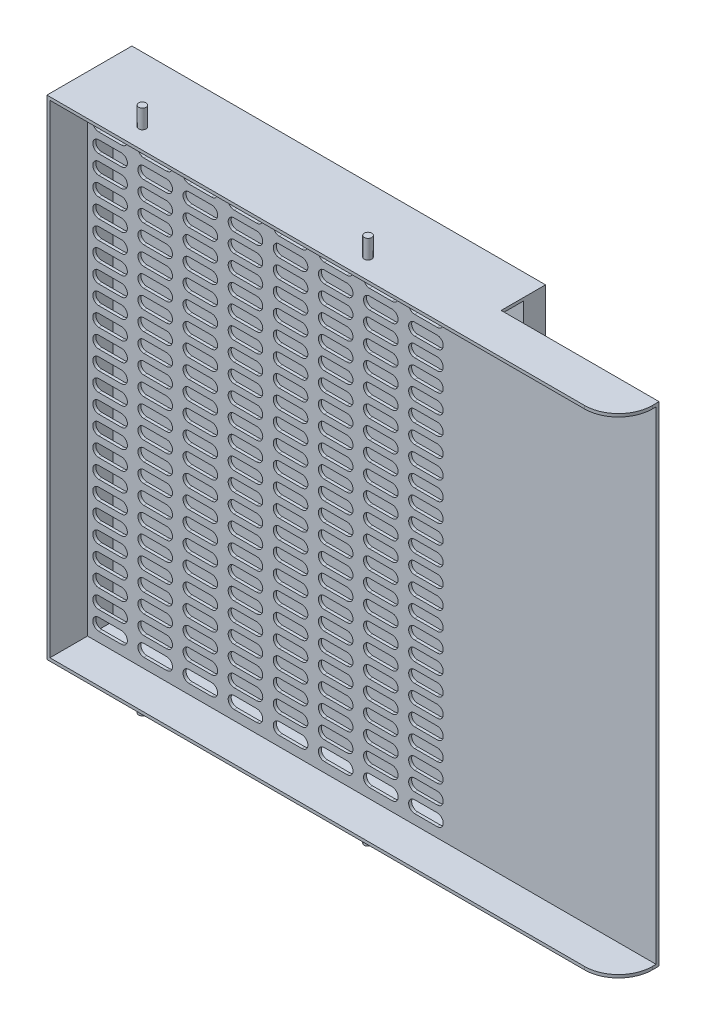
SolidWorks part; units mm, degrees
material "AISI 304"
ref_plane "Front Plane" through (0, 0, 0) normal (0, 0, 1) x (1, 0, 0)
ref_plane "Top Plane" through (0, 0, 0) normal (0, 1, 0) x (1, 0, 0)
ref_plane "Right Plane" through (0, 0, 0) normal (1, 0, 0) x (0, 0, -1)
other "Configuration Table"
sketch "Sketch1" plane through (0, 0, 0) normal (0, 0, 1) x (1, 0, 0)
  line L1 (-250, 325) -> (250, 325)
  line L2 (-250, 325) -> (-250, -325)
  line L3 (-250, -325) -> (250, -325)
  line L4 (250, 325) -> (250, -325)
  line L5 (-250, 325) -> (250, -325) construction
  line L6 (-250, -325) -> (250, 325) construction
  point P0 (0, 0)
  dimension "D1" = 500
  dimension "D2" = 650
extrude "Boss-Extrude1" add sketch "Sketch1" along normal mid plane 4
sketch "Sketch2" plane through (0, 0, 2) normal (0, 0, 1) x (1, 0, 0)
  line L0 (-246, 321) -> (-246, -321)
  line L1 (-246, -321) -> (246, -321)
  line L2 (246, -321) -> (246, 321)
  line L3 (246, 321) -> (-246, 321)
  line L4 (250, -325) -> (250, 325)
  line L5 (250, 325) -> (-250, 325)
  line L6 (-250, 325) -> (-250, -325)
  line L7 (-250, -325) -> (250, -325)
  line L8 (250, -325) -> (250, 325)
  line L9 (250, 325) -> (-250, 325)
  line L10 (-250, 325) -> (-250, -325)
  line L11 (-250, -325) -> (250, -325)
  dimension "D2" = 4
  dimension "D1" = 0
extrude "Boss-Extrude2" add sketch "Sketch2" along normal blind 50
sketch "Sketch3" plane through (0, -325, 0) normal (0, -1, 0) x (1, 0, 0)
  line L0 (-250, 25) -> (250, 25) construction
  line L1 (-250, 52) -> (-250, -2) construction
  line L2 (250, 52) -> (250, -2) construction
  circle A0 centre (150, 25) radius 5
  circle A1 centre (-150, 25) radius 5
  dimension "D1" = 10
  dimension "D2" = 10
  dimension "D3" = 100
  dimension "D4" = 300
extrude "Boss-Extrude3" add sketch "Sketch3" along normal blind 25
sketch "Sketch4" plane through (0, 325, 0) normal (0, 1, 0) x (1, 0, 0)
  line L0 (250, -25) -> (-250, -25) construction
  line L1 (250, -52) -> (250, 2) construction
  line L2 (-250, -52) -> (-250, 2) construction
  circle A0 centre (150, -25) radius 5
  circle A1 centre (-150, -25) radius 5
  dimension "D1" = 10
  dimension "D2" = 10
  dimension "D3" = 300
  dimension "D4" = 100
extrude "Boss-Extrude4" add sketch "Sketch4" along normal blind 25
sketch "Sketch5" plane through (246, 0, 0) normal (-1, 0, 0) x (0, 0, 1)
  line L4 (2, 321) -> (2, -321)
  line L5 (2, -321) -> (52, -321)
  line L6 (52, -321) -> (52, 321)
  line L7 (52, 321) -> (2, 321)
  line L8 (2, 321) -> (2, -321)
  line L9 (2, -321) -> (52, -321)
  line L10 (52, -321) -> (52, 321)
  line L11 (52, 321) -> (2, 321)
  dimension "D1" = 0
extrude "Cut-Extrude1" cut sketch "Sketch5" against normal blind 25
sketch "Sketch6" plane through (250, 0, 0) normal (1, 0, 0) x (0, 0, -1)
  line L8 (-52, 325) -> (-52, 321)
  line L9 (-52, 321) -> (-2, 321)
  line L10 (-2, 321) -> (-2, -321)
  line L11 (-2, -321) -> (-52, -321)
  line L12 (-52, -321) -> (-52, -325)
  line L13 (-52, -325) -> (2, -325)
  line L14 (2, -325) -> (2, 325)
  line L15 (2, 325) -> (-52, 325)
  line L16 (-52, 325) -> (-52, 321)
  line L17 (-52, 321) -> (-2, 321)
  line L18 (-2, 321) -> (-2, -321)
  line L19 (-2, -321) -> (-52, -321)
  line L20 (-52, -321) -> (-52, -325)
  line L21 (-52, -325) -> (2, -325)
  line L22 (2, -325) -> (2, 325)
  line L23 (2, 325) -> (-52, 325)
  dimension "D1" = 0
extrude "Boss-Extrude5" add sketch "Sketch6" along normal blind 50
sketch "Sketch9" plane through (0, 0, -2) normal (0, 0, -1) x (-1, 0, 0)
  line L0 (-296, 321) -> (-296, -321)
  line L1 (-296, -321) -> (246, -321)
  line L2 (246, -321) -> (246, 321)
  line L3 (246, 321) -> (-296, 321)
  line L4 (250, 325) -> (-300, 325)
  line L5 (-300, 325) -> (-300, -325)
  line L6 (-300, -325) -> (250, -325)
  line L7 (250, -325) -> (250, 325)
  line L8 (250, 325) -> (-300, 325)
  line L9 (-300, 325) -> (-300, -325)
  line L10 (-300, -325) -> (250, -325)
  line L11 (250, -325) -> (250, 325)
  line L12 (-296, 321) -> (-300, 321)
  line L13 (-296, -321) -> (-300, -321)
  line M9 (250, 325) -> (-300, 325)
  line M10 (-300, 325) -> (-300, -325)
  line M11 (-300, -325) -> (250, -325)
  line M12 (250, -325) -> (250, 325)
  dimension "D1" = 0
  dimension "D2" = 4
extrude "Boss-Extrude7" add sketch "Sketch9" along normal blind 30 contours L1 L13 L12 L3 L2 M10 M11 M12 M9
sketch "Sketch10" plane through (0, 0, -32) normal (0, 0, -1) x (-1, 0, 0)
  line L1 (-300, 325) -> (250, 325)
  line L2 (-300, 325) -> (-300, -325)
  line L3 (-300, -325) -> (250, -325)
  line L4 (250, 325) -> (250, -325)
extrude "Boss-Extrude8" add sketch "Sketch10" along normal blind 4
sketch "Sketch11" plane through (0, 0, 2) normal (0, 0, 1) x (1, 0, 0)
  line L0 (-246, 0) -> (300, 0) construction
  line L1 (-246, 321) -> (-246, -321) construction
  line L2 (300, 321) -> (300, -321) construction
  line L3 (-231, 0) -> (-201, 0) construction
  line L4 (-231, 8) -> (-201, 8)
  line L5 (-231, -8) -> (-201, -8)
  line L6 (-171, 0) -> (-141, 0) construction
  line L7 (-171, 8) -> (-141, 8)
  line L8 (-171, -8) -> (-141, -8)
  line L9 (-111, 0) -> (-81, 0) construction
  line L10 (-111, 8) -> (-81, 8)
  line L11 (-111, -8) -> (-81, -8)
  line L12 (-51, 0) -> (-21, 0) construction
  line L13 (-51, 8) -> (-21, 8)
  line L14 (-51, -8) -> (-21, -8)
  line L15 (9, 0) -> (39, 0) construction
  line L16 (9, 8) -> (39, 8)
  line L17 (9, -8) -> (39, -8)
  line L18 (69, 0) -> (99, 0) construction
  line L19 (69, 8) -> (99, 8)
  line L20 (69, -8) -> (99, -8)
  line L21 (129, 0) -> (159, 0) construction
  line L22 (129, 8) -> (159, 8)
  line L23 (129, -8) -> (159, -8)
  line L24 (189, 0) -> (219, 0) construction
  line L25 (189, 8) -> (219, 8)
  line L26 (189, -8) -> (219, -8)
  arc A0 (-231, 8) -> (-231, -8) centre (-231, 0) ccw
  arc A1 (-201, -8) -> (-201, 8) centre (-201, 0) ccw
  arc A2 (-171, 8) -> (-171, -8) centre (-171, 0) ccw
  arc A3 (-141, -8) -> (-141, 8) centre (-141, 0) ccw
  arc A4 (-111, 8) -> (-111, -8) centre (-111, 0) ccw
  arc A5 (-81, -8) -> (-81, 8) centre (-81, 0) ccw
  arc A6 (-51, 8) -> (-51, -8) centre (-51, 0) ccw
  arc A7 (-21, -8) -> (-21, 8) centre (-21, 0) ccw
  arc A8 (9, 8) -> (9, -8) centre (9, 0) ccw
  arc A9 (39, -8) -> (39, 8) centre (39, 0) ccw
  arc A10 (69, 8) -> (69, -8) centre (69, 0) ccw
  arc A11 (99, -8) -> (99, 8) centre (99, 0) ccw
  arc A12 (129, 8) -> (129, -8) centre (129, 0) ccw
  arc A13 (159, -8) -> (159, 8) centre (159, 0) ccw
  arc A14 (189, 8) -> (189, -8) centre (189, 0) ccw
  arc A15 (219, -8) -> (219, 8) centre (219, 0) ccw
  point P8 (-216, 0)
  point P16 (-156, 0)
  point P23 (-96, 0)
  point P30 (-36, 0)
  point P37 (24, 0)
  point P44 (84, 0)
  point P51 (144, 0)
  point P58 (204, 0)
  dimension "D2" = 8
  dimension "D1" = 30
  dimension "D3" = 15
  dimension "D4" = 8
extrude "Cut-Extrude3" cut sketch "Sketch11" against normal blind 4
pattern_linear "LPattern1" count 13 spacing 25 along (0, -1, 0) of "Cut-Extrude3"
pattern_linear "LPattern2" count 13 spacing 25 along (0, 1, 0) of "Cut-Extrude3"
sketch "Sketch13" plane through (0, 0, -36) normal (0, 0, -1) x (-1, 0, 0)
  line L0 (-275, 300) -> (-275, -300)
  line L1 (-275, -300) -> (225, -300)
  line L2 (225, -300) -> (225, 300)
  line L3 (225, 300) -> (-275, 300)
  line L4 (-300, 325) -> (-300, -325)
  line L5 (-300, -325) -> (250, -325)
  line L6 (250, -325) -> (250, 325)
  line L7 (250, 325) -> (-300, 325)
  line L8 (-300, 325) -> (-300, -325)
  line L9 (-300, -325) -> (250, -325)
  line L10 (250, -325) -> (250, 325)
  line L11 (250, 325) -> (-300, 325)
  line L13 (300, 31.3075) -> (-300, 31.3075)
  line L14 (300, 31.3075) -> (300, -31.3075)
  line L15 (300, -31.3075) -> (-300, -31.3075)
  line L16 (-300, 31.3075) -> (-300, -31.3075)
  line L17 (300, 31.3075) -> (-300, -31.3075) construction
  line L18 (300, -31.3075) -> (-300, 31.3075) construction
  line L19 (305.8934, 6.3075) -> (-300, 6.3075)
  line L20 (305.8934, 6.3075) -> (305.8934, -5.6925)
  line L21 (305.8934, -5.6925) -> (-300, -5.6925)
  line L22 (-300, 6.3075) -> (-300, -5.6925)
  line L23 (305.8934, 6.3075) -> (-300, -5.6925) construction
  line L24 (305.8934, -5.6925) -> (-300, 6.3075) construction
  point P8 (0, 0)
  point P13 (2.9467, 0.3075)
  line M15 (-300, 325) -> (-300, -325)
  line M16 (-300, -325) -> (250, -325)
  line M17 (250, -325) -> (250, 325)
  line M18 (250, 325) -> (-300, 325)
  dimension "D3" = 25
  dimension "D4" = 605.8934
  dimension "D5" = 12
  dimension "D1" = 0
  dimension "D2" = 25
extrude "Boss-Extrude10" add sketch "Sketch13" along normal blind 25 contours L13 L10 L0 L3 L2 M18 M15 | L19 L2 L13 L0 | L2 L21 L0 L15 | L0 L21 L8 L15 | L19 L0 L13 L8 | L15 L2 L1 L0 M17 M15 M16 | L21 L0 L19 L16 | L10 L21 L2 L15 | L21 L19 L2 M17 | L19 L13 L2 M17
sketch "Sketch14" plane through (0, 0, 0) normal (0, 1, 0) x (1, 0, 0)
  line L0 (-250, 48.5) -> (300, 48.5) construction
  line L1 (-250, -52) -> (-250, 61) construction
  line L2 (300, 61) -> (300, -52) construction
  line L3 (-250, 61) -> (300, 61) construction
  circle A0 centre (25, 48.5) radius 5
  dimension "D2" = 10
  dimension "D1" = 12.5
extrude "Cut-Extrude4" cut sketch "Sketch14" against normal mid plane 80
sketch "Sketch15" plane through (300, 0, 0) normal (1, 0, 0) x (0, 0, -1)
  line L0 (2, 321) -> (2, -325)
  line L1 (2, -325) -> (-52, -325)
  line L2 (2, 320.1324) -> (2, 325)
  line L3 (2, 325) -> (-52, 325)
  line L8 (-52, -325) -> (61, -325)
  line L9 (61, -325) -> (61, 325)
  line L10 (61, 325) -> (-52, 325)
  line L11 (-52, 325) -> (-52, 321)
  line L12 (-52, 321) -> (-2, 321)
  line L13 (-2, 321) -> (-2, -321)
  line L14 (-2, -321) -> (-52, -321)
  line L15 (-52, -321) -> (-52, -325)
  line L16 (-52, -325) -> (61, -325)
  line L17 (61, -325) -> (61, 325)
  line L18 (61, 325) -> (-52, 325)
  line L19 (-52, 325) -> (-52, 321)
  line L20 (-52, 321) -> (-2, 321)
  line L21 (-2, 321) -> (-2, -321)
  line L22 (-2, -321) -> (-52, -321)
  line L23 (-52, -321) -> (-52, -325)
  line M9 (-52, -325) -> (61, -325)
  line M11 (61, 325) -> (-52, 325)
  line M12 (-52, 325) -> (-52, 321)
  line M13 (-52, 321) -> (-2, 321)
  line M14 (-2, 321) -> (-2, -321)
  line M15 (-2, -321) -> (-52, -321)
  line M16 (-52, -321) -> (-52, -325)
  line M19 (2, -321) -> (2, 321)
  dimension "D1" = 0
extrude "Boss-Extrude11" add sketch "Sketch15" along normal blind 210 contours L0 L2 M11 M12 M13 M14 M15 M16 M9 M19
fillet "Fillet1" radius 45 2 edges at (510, 323, 52) (510, -323, 52)
